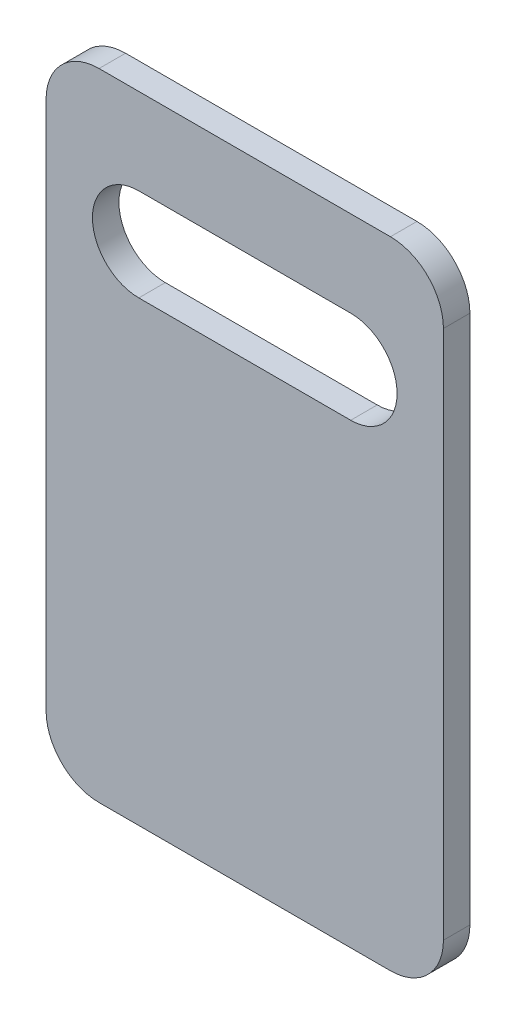
SolidWorks part; units mm, degrees
material "SUS304"
ref_plane "Front Plane" through (0, 0, 0) normal (0, 0, 1) x (1, 0, 0)
ref_plane "Top Plane" through (0, 0, 0) normal (0, 1, 0) x (1, 0, 0)
ref_plane "Right Plane" through (0, 0, 0) normal (1, 0, 0) x (0, 0, -1)
sketch "Sketch1" plane through (0, 0, 0) normal (0, 0, 1) x (1, 0, 0)
  line L0 (-4, 7) -> (4, 7) construction
  line L1 (-7.5, -12) -> (7.5, -12)
  line L2 (-7.5, -12) -> (-7.5, 12)
  line L3 (-7.5, 12) -> (7.5, 12)
  line L4 (7.5, -12) -> (7.5, 12)
  line L5 (-7.5, -12) -> (7.5, 12) construction
  line L6 (-7.5, 12) -> (7.5, -12) construction
  line L7 (-4, 8.75) -> (4, 8.75)
  line L8 (-4, 5.25) -> (4, 5.25)
  line L9 (0, 0) -> (0, 7) construction
  arc A0 (-4, 8.75) -> (-4, 5.25) centre (-4, 7) ccw
  arc A1 (4, 5.25) -> (4, 8.75) centre (4, 7) ccw
  point P0 (0, 0)
  point P8 (0, 7)
  dimension "D1" = 15
  dimension "D2" = 3.5
  dimension "D3" = 8
  dimension "D4" = 5
  dimension "D5" = 24
extrude "Boss-Extrude1" add sketch "Sketch1" along normal blind 1
fillet "Fillet1" radius 2 4 edges at (-7.5, 12, 0.5) (7.5, 12, 0.5) (7.5, -12, 0.5) (-7.5, -12, 0.5)
